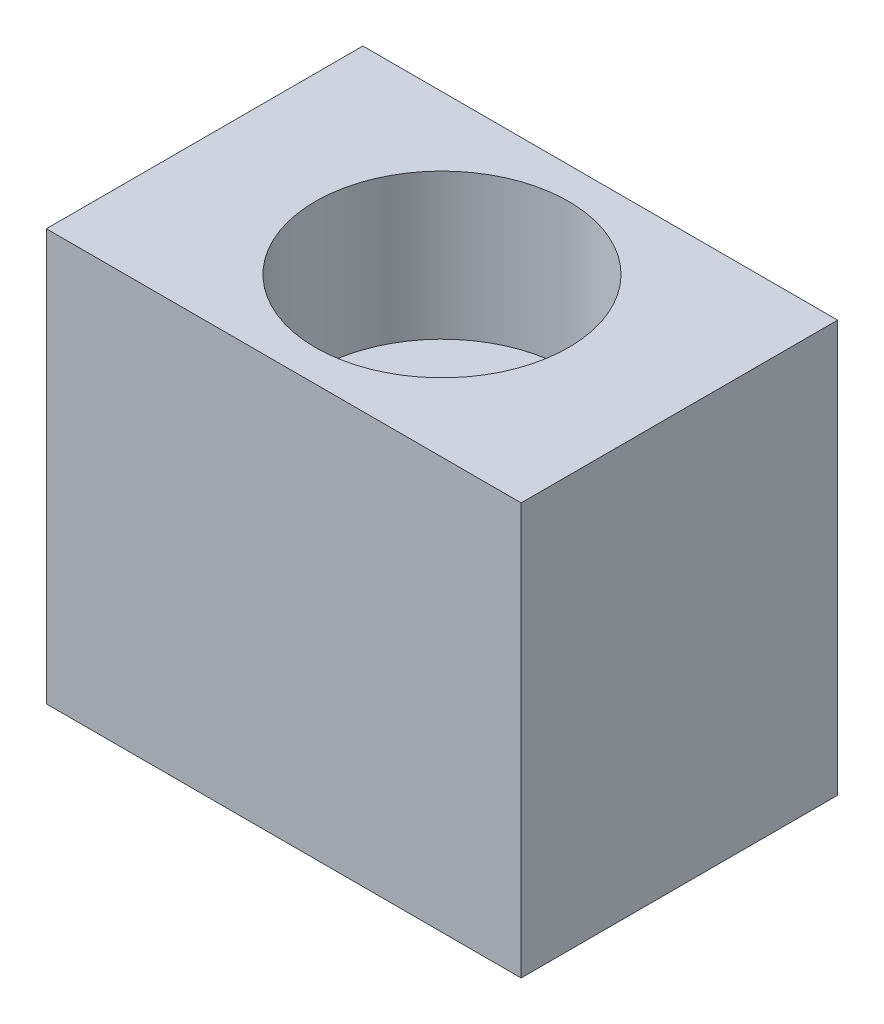
SolidWorks part; units mm, degrees
material "PU "
ref_plane "前基準面" through (0, 0, 0) normal (0, 0, 1) x (1, 0, 0)
ref_plane "上基準面" through (0, 0, 0) normal (0, 1, 0) x (1, 0, 0)
ref_plane "右基準面" through (0, 0, 0) normal (1, 0, 0) x (0, 0, -1)
sketch "草图1" plane through (0, 0, 0) normal (0, 1, 0) x (1, 0, 0)
  line L1 (-7.5, -5) -> (7.5, -5)
  line L2 (-7.5, -5) -> (-7.5, 5)
  line L3 (-7.5, 5) -> (7.5, 5)
  line L4 (7.5, -5) -> (7.5, 5)
  line L5 (-7.5, -5) -> (7.5, 5) construction
  line L6 (-7.5, 5) -> (7.5, -5) construction
  point P0 (0, 0)
  dimension "D1" = 15
  dimension "D2" = 10
extrude "凸台-拉伸1" add sketch "草图1" along normal mid plane 13
hole_wizard "打孔尺寸(%根据)内六角圆柱头螺钉的类型1" positions "草图2" profile "草图3" counterbore size "M4" standard "GB" end condition through all
sketch "草图2" plane through (0, 6.5, 0) normal (0, 1, 0) x (1, 0, 0)
  point P0 (0, 0)
sketch "草图3" plane through (0, 6.5, 0) normal (1, 0, 0) x (0, 0, 1)
  line L0 (0, 0) -> (0, 13)
  line L1 (0, 13) -> (2.25, 13)
  line L3 (2.25, 13) -> (2.25, 4.6)
  line L4 (2.25, 4.6) -> (4, 4.6)
  line L5 (4, 4.6) -> (4, 0)
  line L7 (4, 0) -> (0, 0)
  line L11 (0, -6.35) -> (0, 107.95) construction
  dimension "通孔孔直径" = 4.5
  dimension "通孔孔深度" = 13
  dimension "柱形沉头孔直径" = 8
  dimension "柱形沉头孔深度" = 4.6
